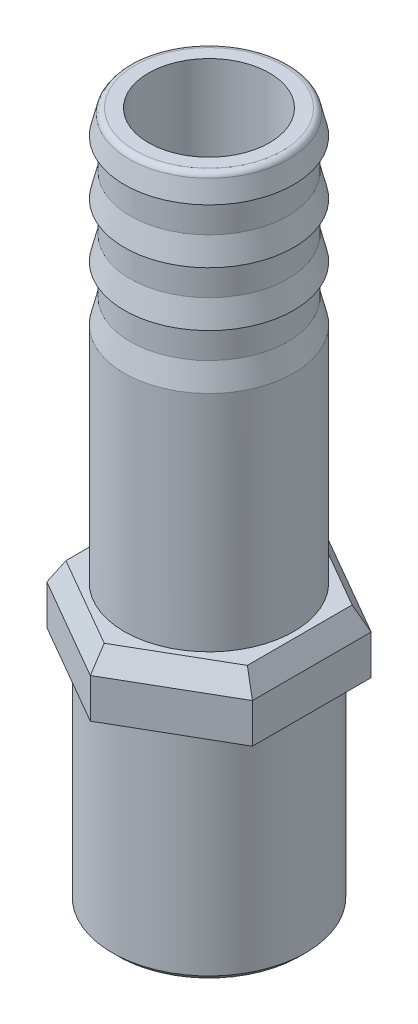
from build123d import *

# Parameters (mm, degrees)
SKETCH2_R           = 7
BOSS_EXTRUDE1_DEPTH = 34
BOSS_EXTRUDE2_DEPTH = 5
SKETCH6_R           = 8
BOSS_EXTRUDE3_DEPTH = 18
SKETCH4_R           = 5
CUT_EXTRUDE1_DEPTH  = 59.460100353
CHAMFER1_SIZE       = 1
CHAMFER1_SIZE2      = 1.732050808
CHAMFER3_SIZE       = 0.5
FILLET1_R           = 0.5


with BuildPart() as part:
    # Sketch2 → Boss-Extrude1 (new body)
    with BuildSketch(Plane(origin=(0, 0, 0), x_dir=(1, 0, 0), z_dir=(0, 1, 0))):
        with Locations(Location((0, 0, 0), (0, 0, 270))):
            Circle(SKETCH2_R)
    extrude(amount=BOSS_EXTRUDE1_DEPTH)

    # Sketch3 → Cut-Revolve1 (revolve, cut)
    with BuildSketch(Plane.XY, mode=Mode.PRIVATE) as cut_revolve1_sk:
        Polygon((6.5, 34), (7, 32), (6.5, 32), (6.5, 29.5), (7, 27.5), (6.5, 27.5), (6.5, 25), (7, 23), (6.5, 23), (6.5, 20.5), (7, 18.5), (7, 34), align=None)
    revolve(cut_revolve1_sk.sketch.rotate(Axis((0, 0, 0), (0, 1, 0)), 90), axis=Axis((0, 0, 0), (0, 1, 0)), mode=Mode.SUBTRACT)

    # Sketch5 → Boss-Extrude2 (add)
    with BuildSketch(Plane.XZ):
        Polygon((8.5, -4.907477288), (8.5, 4.907477288), (0, 9.814954576), (-8.5, 4.907477288), (-8.5, -4.907477288), (0, -9.814954576), align=None)
    extrude(amount=BOSS_EXTRUDE2_DEPTH)

    # Sketch6 → Boss-Extrude3 (add)
    with BuildSketch(Plane.XZ.offset(5)):
        with Locations(Location((0, 0, 0), (0, 0, 270))):
            Circle(SKETCH6_R)
    extrude(amount=BOSS_EXTRUDE3_DEPTH)

    # Sketch4 → Cut-Extrude1 (cut, through all)
    with BuildSketch(Plane(origin=(0, 34, 0), x_dir=(1, 0, 0), z_dir=(0, 1, 0))):
        with Locations(Location((0, 0, 0), (0, 0, 270))):
            Circle(SKETCH4_R)
    extrude(amount=-CUT_EXTRUDE1_DEPTH, mode=Mode.SUBTRACT)

    # Chamfer1
    chamfer1_edges = [part.edges().sort_by_distance(p)[0] for p in [
        (4.25, 0, -7.361215932),
        (8.5, 0, 0),
        (4.25, 0, 7.361215932),
        (-4.25, 0, 7.361215932),
        (-8.5, 0, 0),
        (-4.25, 0, -7.361215932),
    ]]
    chamfer1_side = [part.faces().sort_by_distance(p)[0] for p in [
        (8.240320711, 0, 0),
    ]]
    chamfer(chamfer1_edges, length=CHAMFER1_SIZE, length2=CHAMFER1_SIZE2, reference=chamfer1_side[0])

    # Chamfer3
    chamfer3_edges = [part.edges().sort_by_distance(p)[0] for p in [
        (0, -23, 8),
    ]]
    chamfer(chamfer3_edges, length=CHAMFER3_SIZE)

    # Fillet1
    fillet1_edges = [part.edges().sort_by_distance(p)[0] for p in [
        (0, 34, 6.5),
    ]]
    fillet(fillet1_edges, radius=FILLET1_R)


solid = part.part
